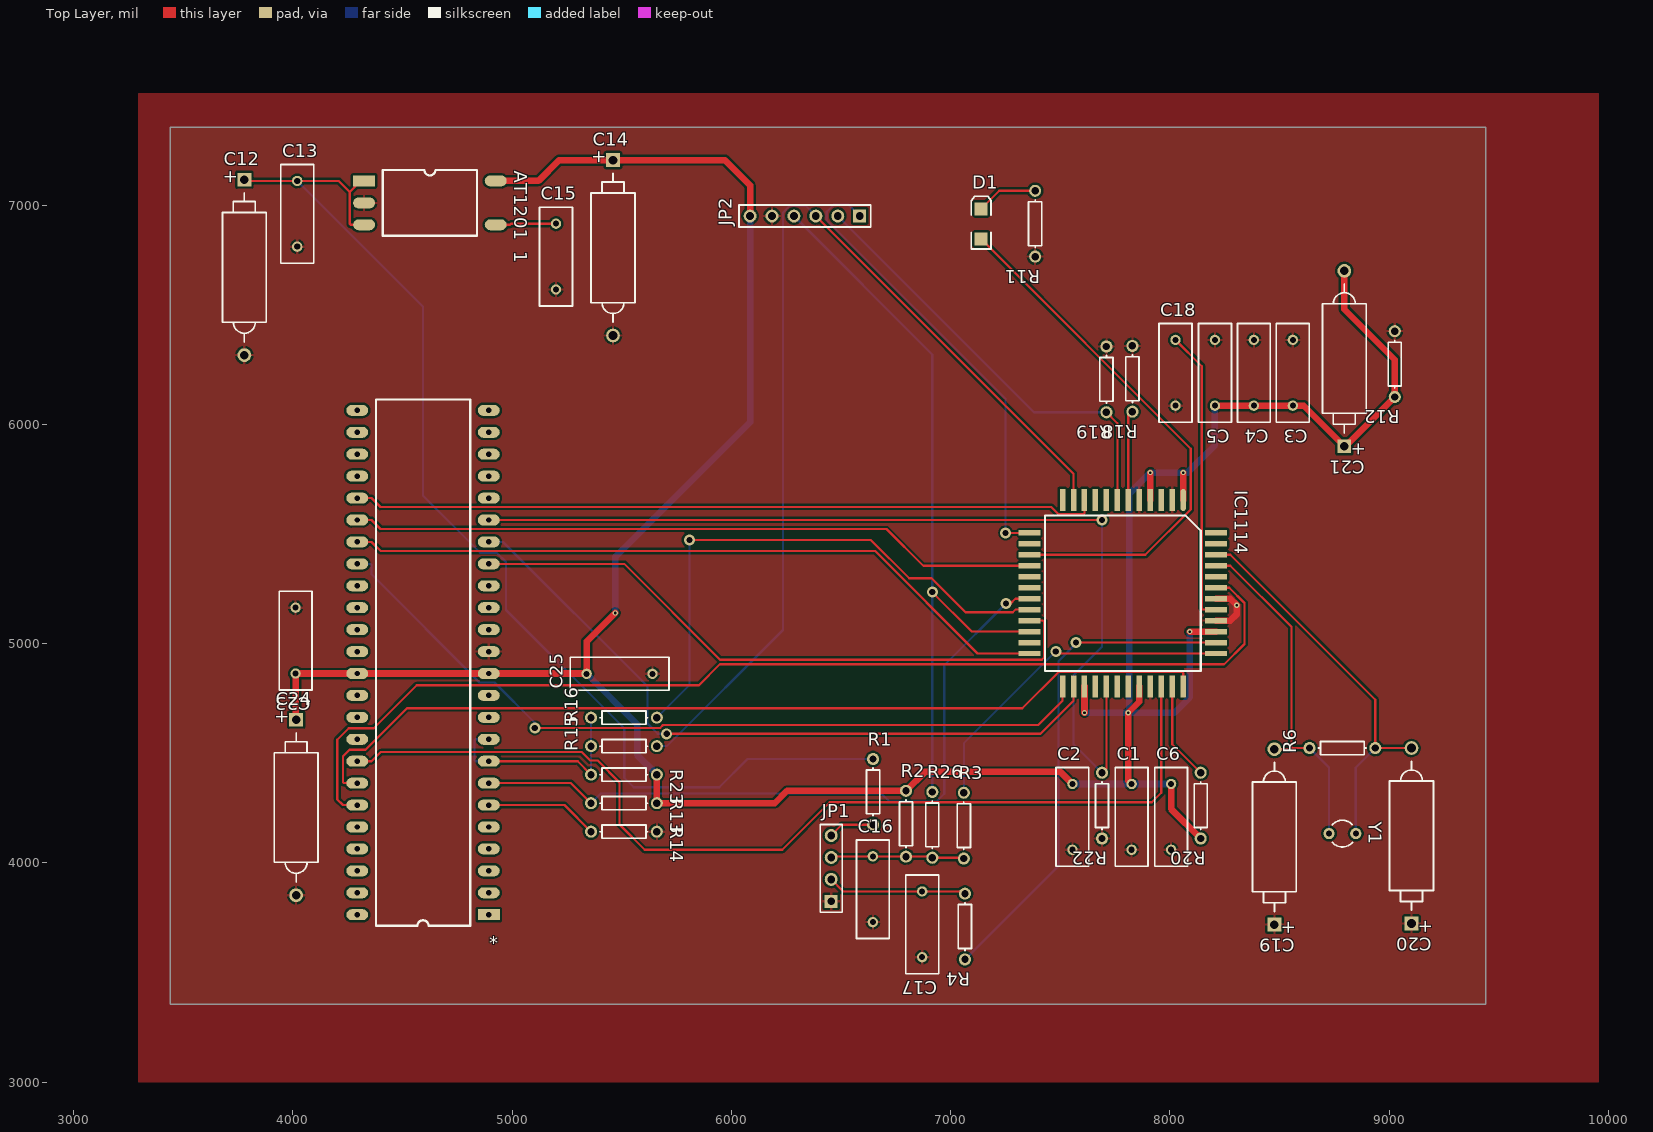
[diagram p0: Top Layer view]
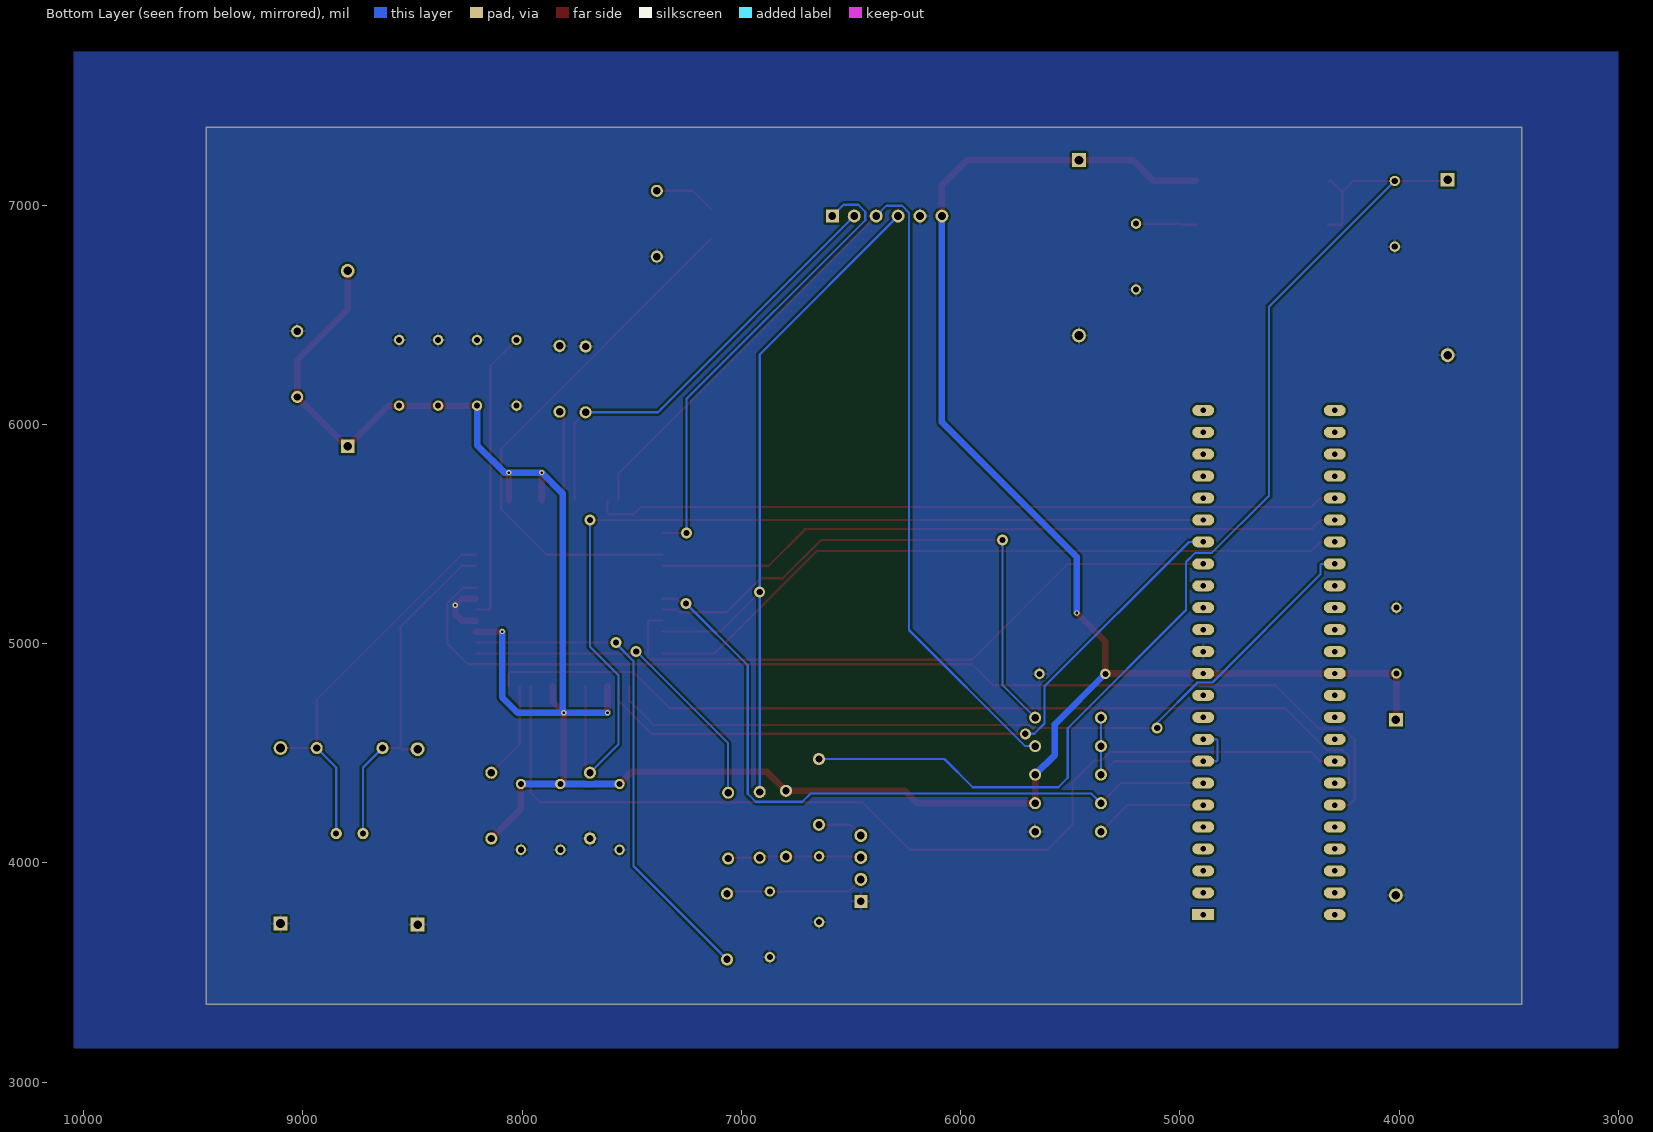
[diagram p1: Bottom Layer view, seen from below]
# Altium PCB MISC75231.pcbdoc
Units mil, origin at the board's own origin, x right, y up, seen from the top; angles counter-clockwise.
Board outline 6000 x 4000 mil, 2 copper layers (Top Layer, Bottom Layer); 43 components, 44 nets, 187 pads, 16 vias.

## Layer stack, top to bottom (the 12.6 mil dielectric is the usual default, probably not edited)
Top Solder Mask Layer: solder mask 0.4, Solder Resist, Dk 3.5
Top Layer: signal copper 1.4
Dielectric 1: surface 12.6, FR-4, Dk 4.8
Bottom Layer: signal copper 1.4
Bottom Solder Mask Layer: solder mask 0.4, Solder Resist, Dk 3.5

## Board outline
3440,7355 3440,3355 9440,3355 9440,7355

## Design rules (kind name [scope] priority, off if disabled: settings)
BoardOutlineClearance Clearance_1 [All] p2: genericclearance=10 ignorepadtopadclearanceinfootprint=FALSE except(0: Arc-SplitContinuation Track-SplitContinuation SMDPad-SplitContinuation THPad-SplitContinuation Via-SplitContinuation Fill-SplitContinuation Region-SplitContinuation Poly-SplitContinuation Text-SplitContinuation Hole-SplitContinuation; 6: SMDPad-CutoutEdge THPad-CutoutEdge Via-CutoutEdge Fill-CutoutEdge Region-CutoutEdge Text-CutoutEdge; 6.9: Hole-CutoutEdge; 10: Arc-OutlineEdge Track-OutlineEdge SMDPad-OutlineEdge THPad-OutlineEdge Via-OutlineEdge Fill-OutlineEdge Region-OutlineEdge Poly-OutlineEdge Text-OutlineEdge Hole-OutlineEdge Poly-CutoutEdge; 11.8: Arc-CutoutEdge Track-CutoutEdge)
Clearance [All] p1: gap=10 ignorepadtopadclearanceinfootprint=FALSE
DiffPairsRouting [All] p1: maxlimit=10 minlimit=6 mostfreqgap=6 toplayer_minwidth=15 toplayer_prefwidth=15 toplayer_maxwidth=15 toplayer_mingap=10 toplayer_prefgap=10 toplayer_maxgap=10 bottomlayer_minwidth=15 bottomlayer_prefwidth=15 bottomlayer_maxwidth=15 bottomlayer_mingap=10 bottomlayer_prefgap=10 bottomlayer_maxgap=10 maxuncoupledlength=10
HoleToHoleClearance ComponentClearance [All] p1: gap=10 allowstackedmicrovias=TRUE
Length netLength [All] p1: minlimit=0 maxlimit=0
MatchedLengths netLengthTolerance [All] p1: tolerance=1000
PolygonConnect [(InNet('GND'))] p1: connectstyle=Relief reliefconductorwidth=10 reliefentries=4 polygonreliefangle="90 Angle" airgapwidth=10 via.connectstyle=Relief via.reliefconductorwidth=10 via.reliefentries=4 via.polygonreliefangle="90 Angle" via.airgapwidth=10
RoutingVias [All] p1: holewidth=28 width=50 viastyle="Through Hole" minholewidth=28 minwidth=50 maxholewidth=28 maxwidth=50
SolderMaskExpansion [All] p1: expansion=4 istentingtop=FALSE
Width [All] p1: maxlimit=10 minlimit=10 preferedwidth=10 toplayer_minwidth=5 toplayer_maxwidth=100 toplayer_prefwidth=10 bottomlayer_minwidth=5 bottomlayer_maxwidth=100 bottomlayer_prefwidth=10
2 further rules are at their usual default settings.

## Components (designator, comment, footprint, x,y, rotation, side; value= is the part's Value field where it differs from the comment)
* "Component_2" DIP48 4893.6,3763.78 r180 top
"AT1201  1" "AT1201_SOT25" SOP6 4325,7110 r0 top
C1 "" RAD-0.3 7825,4210 r90 top
C2 "" RAD-0.3 7555,4210 r90 top
C3 "" RAD-0.3 8560,6235 r270 top
C4 "" RAD-0.3 8382.5,6235 r270 top
C5 "" RAD-0.3 8205,6235 r270 top
C6 "" RAD-0.3 8005,4210 r90 top
C12 "" POLAR0.8 3778.82,6715.75 r90 top
C13 "" RAD-0.3 4020,6960 r90 top
C14 "" POLAR0.8 5460,6805 r90 top
C15 "" RAD-0.3 5200,6765 r90 top
C16 "" RAD-0.3 6645,3880 r90 top
C17 "" RAD-0.3 6870,3720 r270 top
C18 "" RAD-0.3 8025,6235 r90 top
C19 "" POLAR0.8 8476.22,4118.78 r270 top
C20 "" POLAR0.8 9101.22,4123.78 r270 top
C21 "" POLAR0.8 8795,6300 r270 top
C23 "" RAD-0.3 4012.42,5013.78 r270 top
C24 "" POLAR0.8 4015,4252.56 r90 top
C25 "" RAD-0.3 5490,4862.56 r180 top
D1 "LED2" 3.2X1.6X1.1 7138.84,6913.78 r90 top
IC1114 "Component_1" Quad48 8060,5655 r270 top
JP1 "Header 4" HDR1X4 6455,3825 r90 top
JP2 "JUMPER6_1.27MM" HDR1X6 6585,6950 r180 top
R1 "Res1" AXIAL-0.3 6645.93,4323.78 r90 top
R2 "" AXIAL-0.3 6796.04,4178.78 r90 top
R3 "" AXIAL-0.3 7060,4170 r90 top
R4 "" AXIAL-0.3 7065,3710 r270 top
R6 "" AXIAL-0.3 8786.22,4523.78 r180 top
R11 "" AXIAL-0.3 7385,6915 r270 top
R12 "" AXIAL-0.3 9025,6275 r270 top
R13 "" AXIAL-0.3 5510,4272.56 r0 top
R14 "" AXIAL-0.3 5510,4142.56 r0 top
R15 "" AXIAL-0.3 5510,4532.56 r180 top
R16 "" AXIAL-0.3 5510,4662.56 r180 top
R18 "" AXIAL-0.3 7828.6,6207.72 r270 top
R19 "" AXIAL-0.3 7710,6205 r270 top
R20 "" AXIAL-0.3 8140,4261.38 r270 top
R22 "" AXIAL-0.3 7690,4261.38 r270 top
R23 "" AXIAL-0.3 5510,4402.56 r0 top
R26 "" AXIAL-0.3 6916.04,4173.78 r90 top
Y1 "" R38 8786.22,4133.78 r270 top

## Footprints (in the part's own frame and the unit in brackets; to place one, negate y for a bottom-side part, rotate by r counter-clockwise, add the part's x,y. Pads: shape width x height; smd on the part's side, far side on the other; paste and mask are expansions set on the pad)
3.2X1.6X1.1 [mm]
  rect 1.5x1.5 smd: 1(-1.75,0) 2(1.75,0)
  silkscreen extent -2.9,-1.15 3.2,1.15
AXIAL-0.3 [mm]
  round 1.4 hole 0.85: 1(-3.81,0) 2(3.81,0)
  silkscreen extent -2.77,-0.76 2.77,0.76
DIP48 [mil]
  rect 100x50 hole 25: 1(0,0)
  oval 100x50 hole 25: 2(0,-100) 3(0,-200) 4(0,-300) 5(0,-400) 6(0,-500) 7(0,-600) 8(0,-700) 9(0,-800) 10(0,-900) 11(0,-1000) 12(0,-1100) 13(0,-1200) 14(0,-1300) 15(0,-1400) 16(0,-1500) 17(0,-1600) 18(0,-1700) 19(0,-1800) 20(0,-1900) 21(0,-2000) 22(0,-2100) 23(0,-2200) 24(0,-2300) 25(600,-2300) 26(600,-2200) 27(600,-2100) 28(600,-2000) 29(600,-1900) 30(600,-1800) 31(600,-1700) 32(600,-1600) 33(600,-1500) 34(600,-1400) 35(600,-1300) 36(600,-1200) 37(600,-1100) 38(600,-1000) 39(600,-900) 40(600,-800) 41(600,-700) 42(600,-600) 43(600,-500) 44(600,-400) 45(600,-300) 46(600,-200) 47(600,-100) 48(600,0)
  silkscreen extent 85,-2350 515,50
HDR1X4 [mm]
  rect 1.5x1.5 hole 0.9: 1(0,0)
  round 1.5 hole 0.9: 2(2.54,0) 3(5.08,0) 4(7.62,0)
  silkscreen extent -1.27,-1.27 8.89,1.27
HDR1X6 [mm]
  rect 1.5x1.5 hole 0.9: 1(0,0)
  round 1.5 hole 0.9: 2(2.54,0) 3(5.08,0) 4(7.62,0) 5(10.16,0) 6(12.7,0)
  silkscreen extent -1.27,-1.27 13.97,1.27
POLAR0.8 [mm]
  rect 1.6x1.6 hole 1: 1(10.16,0)
  round 1.6 hole 1: 2(-10.16,0)
  silkscreen extent -8.64,-2.54 8.64,2.54
Quad48 [mil]
  oval 100x25 smd: 1(0,0)
  rect 100x25 smd: 2(0,-50) 3(0,-100) 4(0,-150) 5(0,-200) 6(0,-250) 7(0,-300) 8(0,-350) 9(0,-400) 10(0,-450) 11(0,-500) 12(0,-550) 25(850,-550) 26(850,-500) 27(850,-450) 28(850,-400) 29(850,-350) 30(850,-300) 31(850,-250) 32(850,-200) 33(850,-150) 34(850,-100) 35(850,-50) 36(850,0)
  rect 25x100 smd: 13(150,-700) 14(200,-700) 15(250,-700) 16(300,-700) 17(350,-700) 18(400,-700) 19(450,-700) 20(500,-700) 21(550,-700) 22(600,-700) 23(650,-700) 24(700,-700) 37(700,150) 38(650,150) 39(600,150) 40(550,150) 41(500,150) 42(450,150) 43(400,150) 44(350,150) 45(300,150) 46(250,150) 47(200,150) 48(150,150)
  silkscreen extent 70,-630 780,80
R38 [mm]
  round 1.3 hole 0.7: 1(0,1.55) 2(0,-1.55)
  silkscreen extent -1.55,-1.19 1.55,1.17
RAD-0.3 [mm]
  round 1.2 hole 0.7: 1(-3.81,0) 2(3.81,0)
  silkscreen extent -5.71,-1.91 5.71,1.91
SOP6 [mil]
  rect 100x50 smd: 1(0,0)
  oval 100x50 smd: 2(0,-100) 3(0,-200) 4(600,-200) 5(600,0)
  silkscreen extent 85,-250 515,50

## Via types
v1: diameter 50, hole 28, Top Layer to Bottom Layer, 9 vias
v2: diameter 24.02, hole 12, Top Layer to Bottom Layer, 7 vias

## Nets (pads, with @x,y where several pads share a name; then routed paths per layer and width w, separated by ;. In a path a pad name is that pad's centre, name@x,y a point inside that pad or via, vN(x,y) a via of type N, cw(c..) or ccw(c..) an arc to the next point about the centre after c; other vN are vias at no path point)
$2N3: "AT1201  1.4" C15.2 | length 277.1
  Top Layer w10: 4924.99,6910 4990.16,6910 4995.16,6915 C15.2
$2N34: *.6 R14.1 | length 516.6
  Top Layer w10: *.6 5238.78,4263.78 R14.1
$2N37: *.8 *.9 R15.2 R16.2 R23.1 | length 976.7
  Top Layer w10: *.8 5298.78,4463.77 R23.1
  Bottom Layer w10: *.8 4833.01,4463.77 4828.43,4468.35 4828.43,4559.19 4833.01,4563.77 *.9 ; R23.1 R15.2 R16.2
$2N63: IC1114.12
$2N65: D1.1 IC1114.15 | length 2448.9
  Top Layer w10: D1.1 8094.31,5889.41 8094.31,5611.65 7887.66,5405 IC1114.15
$2N66: D1.2 R11.1 | length 280.3
  Top Layer w10: D1.2 7221.16,7065 R11.1
$2N76: IC1114.37 R3.2 | length 1553.3
  Top Layer w10: v1(7479.26,4964.84) 7489.1,4955 IC1114.37
  Bottom Layer w10: R3.2 7060,4545.58 v1(7479.26,4964.84)
$2N77: IC1114.48
$2N81: C20.2 IC1114.46 R6.1 Y1.1 | length 1812.1
  Top Layer w10: IC1114.46 8275.17,5405 8936.22,4743.94 R6.1 C20.2
  Bottom Layer w10: Y1.1 8847.24,4434.79 R6.1
$2N88: C18.2 IC1114.41 | length 1342.1
  Top Layer w10: C18.2 8144.83,6265.17 8144.83,5159.58 8149.41,5155 IC1114.41
$2N90: IC1114.38 R4.2 | length 2293.2
  Top Layer w10: v1(7571.66,5005) IC1114.38
  Bottom Layer w10: R4.2 7491.33,3986.33 7491.33,4920.1 7571.66,5000.43 v1(7571.66,5005)
$2N93: C17.1 JP1.2 R4.1 | length 636.9
  Top Layer w10: JP1.2 6510,3870 C17.1 7055,3870 R4.1
$2N94: C16.2 JP1.3 R2.1 R3.1 R26.1 | length 611.3
  Top Layer w10: JP1.3 6459.39,4029.39 C16.2@6645,4029.39 ; C16.2 C16.2@6645,4029.39 ; R3.1 7056.22,4023.78 R26.1 6911.04,4028.78 R2.1 6645.61,4028.78 C16.2@6645,4029.39
$2N97: JP1.4 R1.1 | length 211.1
  Top Layer w10: JP1.4 6503.78,4173.78 R1.1
BDA: IC1114.22 JP2.4 R26.2 | length 3406.1
  Top Layer w10: v1(6916.04,5234.94) 7095.98,5055 IC1114.22
  Bottom Layer w10: JP2.4 6916.04,6318.96 v1(6916.04,5234.94) R26.2
GND: "AT1201  1.2" *.13 C1.1 C2.1 C3.1 C4.1 C5.1 C6.1 C12.2 C13.1 C14.2 C15.1 C16.1 C17.2 C18.1 C19.1 C20.1 C23.1 C24.2 C25.1 IC1114.2 IC1114.5 IC1114.33 IC1114.40 IC1114.42 JP1.1 JP2.5 R11.2 R12.1 R14.2 R18.1 R19.1 R22.2 | length 254.9
  Top Layer w30: IC1114.40 8275,5105 8305,5135 v2(8305,5175) 8275,5205 IC1114.42
P11: IC1114.23
P35: IC1114.30
RESET: IC1114.3
SCL: IC1114.11 JP2.3 R15.1 | length 4661.2
  Top Layer w10: JP2.3 7560,5775 IC1114.11
  Bottom Layer w10: R15.1 5705.41,4532.55 6235,5062.14 6235,6964.99 6266.5,6996.49 6338.51,6996.49 JP2.3
SM-CLE: IC1114.31
SM_ALE: *.17 IC1114.21 | length 2947.8
  Top Layer w10: *.17 5511.23,5363.77 5948.33,4926.67 7415.62,4926.67 7425.17,4936.22 7425.17,5100.42 7420.59,5105 IC1114.21
SM_CLE: *.16
SM_EN1: IC1114.20 R16.1 | length 2565.4
  Top Layer w10: v1(5808.26,5472.93) 6635.63,5472.93 6810.73,5297.83 6912.67,5297.83 7067.8,5142.7 7282.53,5142.7 7294.83,5155 IC1114.20
  Bottom Layer w10: R16.1 5808.26,4810.81 v1(5808.26,5472.93)
SM_RDY: *.7 IC1114.19 R13.1 | length 3264.8
  Top Layer w10: *.7 5268.78,4363.77 R13.1 ; v1(7252.2,5182.88) 7272.71,5182.88 7294.83,5205 IC1114.19
  Bottom Layer w10: R13.1 5403.83,4316.39 6683.76,4316.39 6721.48,4278.67 6933.76,4278.67 6970.88,4315.78 6970.88,4901.56 v1(7252.2,5182.88)
SM_WE: *.18 IC1114.26 | length 3255.9
  Top Layer w10: v1(5704.91,4588.86) 7409.03,4588.86 7560,4739.83 IC1114.26
  Bottom Layer w10: *.18 4958.77,5463.77 5617.27,4805.27 5617.27,4635.61 5664.02,4588.86 v1(5704.91,4588.86)
SM_WP: *.19 IC1114.29 R22.1 | length 4458.4
  Top Layer w10: *.19 v1(7690,5563.77) ; R22.1 7710,4431.37 IC1114.29
  Bottom Layer w10: R22.1 7560,4541.38 7560,4855.67 7690,4985.67 v1(7690,5563.77)
SMD0: *.29 IC1114.10 | length 3409.5
  Top Layer w10: *.29 4358.78,5663.77 4399.61,5622.93 7458.12,5622.93 7491.22,5589.83 7605.42,5589.83 7610,5594.41 IC1114.10
SMD1: *.30 IC1114.16 | length 3152.9
  Top Layer w10: *.30 4358.78,5563.77 4399.61,5522.93 6707.4,5522.93 6875.33,5355 IC1114.16
SMD2: *.31 IC1114.24 | length 3277.1
  Top Layer w10: *.31 4358.78,5463.77 4399.61,5422.93 6654.57,5422.93 7122.5,4955 IC1114.24
SMD3: *.32 IC1114.25 | length 3681.9
  Top Layer w10: v1(5103.38,4615.8) 5675.05,4615.8 5688.28,4629.03 7399.2,4629.03 7510,4739.83 IC1114.25
  Bottom Layer w10: *.32 4354.2,5363.77 4358.78,5359.19 4358.78,5315.81 4851.62,4822.96 4919.68,4822.96 5103.38,4639.26 v1(5103.38,4615.8)
SMD4: *.41 IC1114.34 | length 4573.6
  Top Layer w10: *.41 4358.78,4463.77 4400.74,4505.74 5317.14,4505.74 5355.91,4466.97 5390,4466.97 5490,4366.97 5490,4175 5605,4060 6231.48,4060 6447.85,4276.38 7916.38,4276.38 7960,4320 IC1114.34
SMD5: *.42 IC1114.36 | length 4237.9
  Top Layer w10: *.42 4233.02,4363.77 4228.44,4368.35 4228.44,4486 4258.18,4515.74 4331.22,4515.74 4520.75,4705.28 7326.33,4705.28 7491.22,4870.17 8055.42,4870.17 8060,4865.59 IC1114.36
SMD6: *.43 IC1114.43 | length 5037.8
  Top Layer w10: *.43 4228.44,4263.78 4202.71,4289.51 4202.71,4561.94 4254.54,4613.77 4368.58,4613.77 4564.8,4810 5851.71,4810 5947.27,4905.56 8246.84,4905.56 8340,4998.73 8340,5185.59 8270.59,5255 IC1114.43
SMD7: *.44
TM1: IC1114.6 R18.2 | length 410.4
  Top Layer w10: IC1114.6 7810,6039.11 R18.2
TM2: IC1114.7 JP2.2 R19.2 | length 2016.4
  Top Layer w10: R19.2 7760,6005 IC1114.7
  Bottom Layer w10: JP2.2 7380,6055 R19.2
TM3: IC1114.35 R20.1 | length 447.5
  Top Layer w10: IC1114.35 8010,4541.37 R20.1
TM4: IC1114.28
TM5: IC1114.13 JP2.1 | length 2096.1
  Top Layer w10: v1(7250.52,5505) IC1114.13
  Bottom Layer w10: JP2.1 6533.81,7001.19 6466.7,7001.19 6435,6969.49 6435,6930.94 7250.52,6115.42 v1(7250.52,5505)
VCC: "AT1201  1.5" *.12 *.37 C1.2 C2.2 C3.2 C4.2 C5.2 C6.2 C14.1 C21.1 C21.2 C23.2 C24.1 C25.2 IC1114.1 IC1114.4 IC1114.27 IC1114.32 IC1114.39 JP2.6 R2.2 R12.2 R13.2 R20.2 R23.2 | length 13850.4
  Top Layer w30: C24.1 4012.42,4655.14 C23.2 *.37 *.12 5338.78,4863.78 C25.2 5340,5010 v2(5470,5140) ; 4925,7110 5120,7110 5215,7205 C14.1 5970,7205 6085,7090 JP2.6 ; R23.2 R13.2 6197.56,4272.56 6253.78,4328.78 R2.2 6882.26,4415 7500,4415 C2.2 ; v2(7610,4685) IC1114.27 ; C1.2 7810,4375 v2(7810,4685) 7860,4735 IC1114.32 ; IC1114.4 v2(7910,5780) ; C6.2 8005,4246.38 R20.2 ; IC1114.1 v2(8060,5780) ; v2(8090,5055) IC1114.39 ; C5.2 C4.2 C3.2 8610,6085 C21.1 8800,5900 R12.2 9025,6295 8795,6525 C21.2
  Bottom Layer w30: C25.2 5570,4632.56 5570,4492.56 R23.2 ; v2(5470,5140) 5470,5395 6085,6010 JP2.6 ; C2.2 7667.05,4360 7668.23,4358.82 7711.77,4358.82 7712.95,4360 C1.2 C6.2 ; v2(7610,4685) v2@7805,4685 ; v2(7810,4685) 8020,4685 8090,4755 v2(8090,5055) ; 7815,4700 7815,5685 v2(7910,5780) v2(8060,5780) 8080,5780 8205,5905 C5.2
VUSB: "AT1201  1.1" "AT1201  1.3" C12.1 C13.2 R1.2 | length 5392.2
  Top Layer w10: C12.1 3784.57,7110 C13.2 4209.66,7110 4259.83,7059.83 ; 4325,6910 4264.41,6910 4259.83,6914.58 4259.83,7059.83 ; 4325,7110 4310,7110 4259.83,7059.83
  Bottom Layer w10: C13.2 4593.6,6536.39 4593.6,5674.11 4853.94,5413.77 4930.25,5413.77 4971.81,5372.21 4971.81,5153.67 5511.63,4613.86 5511.63,4388.37 5555,4345 5944.86,4345 6073.63,4473.77 R1.2
X1: IC1114.44
X2: C19.2 IC1114.45 R6.2 Y1.2 | length 1600.7
  Top Layer w10: IC1114.45 8275.17,5355 8553.72,5076.44 8553.72,4523.77 ; C19.2 8548.72,4518.77 8553.72,4523.77 ; R6.2 8553.72,4523.77
  Bottom Layer w10: R6.2 8725.2,4434.79 Y1.2
pads on no net: *.1 *.2 *.3 *.4 *.5 *.10 *.11 *.14 *.15 *.20 *.21 *.22 *.23 *.24 *.25 *.26 *.27 *.28 *.33 *.34 *.35 *.36 *.38 *.39 *.40 *.45 *.46 *.47 *.48 IC1114.8 IC1114.9 IC1114.14 IC1114.17 IC1114.18 IC1114.47

## Polygon pours and split planes (outlines as drawn)
GND on Top Layer (solid, remove dead copper, pour order 0): 3295,7510 3295,3000 9955,3000 9955,7510
GND on Bottom Layer (solid, remove dead copper, pour order 2): 3000,7700 3000,3155 10045,3155 10045,7700

## Silkscreen, mask and mechanical layers (free items; w line width, h text height)
Mechanical Layer:
  lines w10: 9390,7350 9395,7355 3445,7355 3445,3380 3460,3365 9420,3365 9420,7345